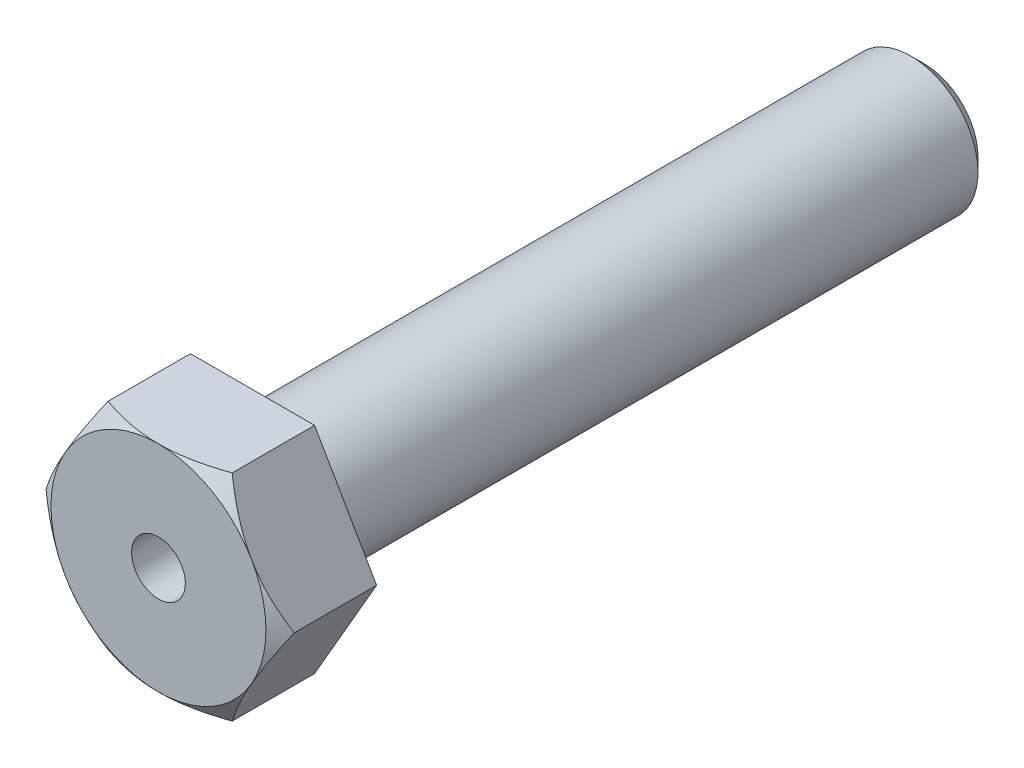
SolidWorks part; units mm, degrees
ref_plane "Front Plane" through (0, 0, 0) normal (0, 0, 1) x (1, 0, 0)
ref_plane "Top Plane" through (0, 0, 0) normal (0, 1, 0) x (1, 0, 0)
ref_plane "Right Plane" through (0, 0, 0) normal (1, 0, 0) x (0, 0, -1)
sketch "Sketch1" plane through (0, 0, 0) normal (1, 0, 0) x (0, 0, -1)
  line L0 (-3.5, 0) -> (25, 0) construction
  line L1 (-3.5, 0) -> (-3.5, 4)
  line L2 (-3.5, 4) -> (0, 4)
  line L3 (0, 4) -> (0, 2.5)
  line L4 (0, 2.5) -> (25, 2.5)
  line L5 (25, 2.5) -> (25, 0)
  point P10 (25, 1)
  dimension "A" = 8
  dimension "E" = 3.5
  dimension "L" = 25
  dimension "M" = 5
  dimension "(d)" = 2
sketch "Sketch3" plane through (0, 0, 0) normal (1, 0, 0) x (0, 0, -1)
  line L2 (0, 2.5) -> (25, 2.5) construction
  line L4 (0, 2.5) -> (-3.5, 2.5)
  line L5 (25, 2.5) -> (25, 0) construction
  line L6 (-3.5, 2.5) -> (-3.5, 1)
  line L8 (0, 2.5) -> (25, 2.5)
  line L10 (25, 1) -> (-3.5, 1)
  line L11 (25, 2.5) -> (25, 1)
revolve "Revolve1" add sketch "Sketch3" angle 360 about L0
cosmetic thread "Cosmetic Thread1" parameters "D1"=25, "D2"=4.25
sketch "Sketch4" plane through (0, 0, 3.5) normal (0, 0, 1) x (1, 0, 0)
  line L7 (2.3094, 4) -> (-2.3094, 4)
  line L8 (-2.3094, 4) -> (-4.6188, 0)
  line L9 (-4.6188, 0) -> (-2.3094, -4)
  line L10 (-2.3094, -4) -> (2.3094, -4)
  line L11 (2.3094, -4) -> (4.6188, 0)
  line L12 (4.6188, 0) -> (2.3094, 4)
  circle A0 centre (0, 0) radius 4 construction
  circle A1 centre (0, 0) radius 1
extrude "Boss-Extrude1" add sketch "Sketch4" against normal up to vertex (3.5 mm away) up to point (0, 4, 0)
sketch "Sketch5" plane through (0, 0, 3.5) normal (0, 0, 1) x (1, 0, 0)
  line L0 (-4, 0) -> (-4.6188, 0) construction
  line L1 (-4.6188, 0) -> (-5.2376, 0) construction
  circle A0 centre (0, 0) radius 4
  circle A1 centre (0, 0) radius 5.2376
  circle A2 centre (0, 0) radius 4 construction
extrude "Cut-Extrude1" cut sketch "Sketch5" against normal blind 1 draft 55
chamfer "Chamfer1" distance 0.5 angle 45 1 edges at (0, -2.5, -25)
